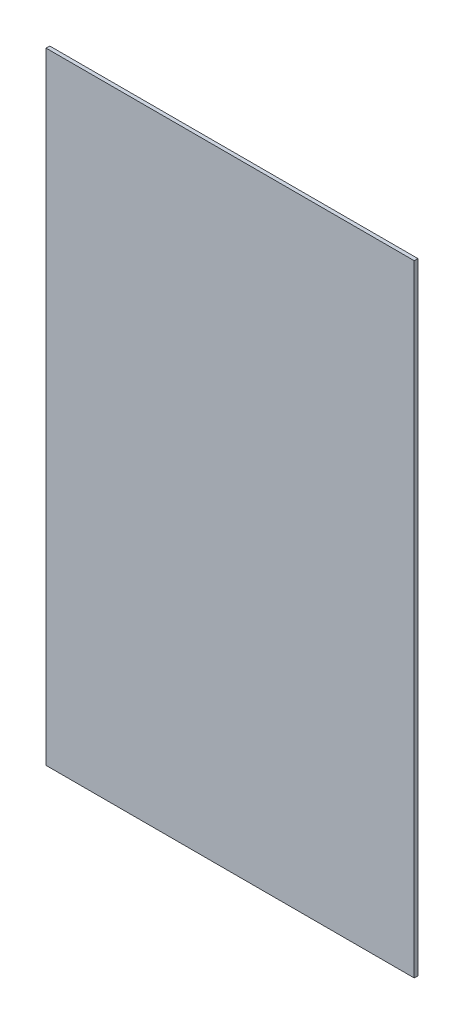
from build123d import *

# Parameters (mm, degrees)
SKETCH_1_W      = 499
SKETCH_1_H      = 842
EXTRUDE_1_DEPTH = 5


with BuildPart() as part:
    # 草图1 → 凸台-拉伸1 (new body)
    with BuildSketch(Plane.XY):
        Rectangle(SKETCH_1_W, SKETCH_1_H)
    extrude(amount=EXTRUDE_1_DEPTH)


solid = part.part
